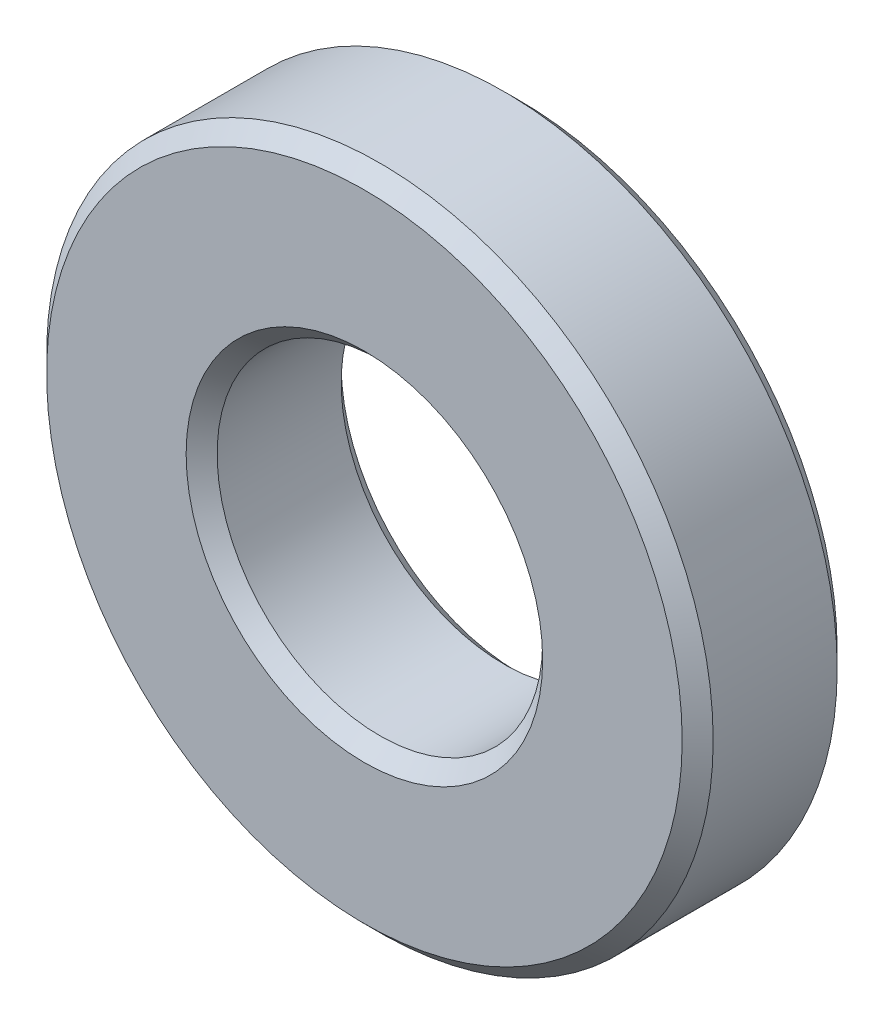
from build123d import *

# Parameters (mm, degrees)
SKETCH1_R           = 10.75
SKETCH1_R_2         = 5.25
BOSS_EXTRUDE1_DEPTH = 5
CHAMFER1_SIZE       = 0.5


with BuildPart() as part:
    # Sketch1 → Boss-Extrude1 (new body)
    with BuildSketch(Plane.XY):
        Circle(SKETCH1_R)
        Circle(SKETCH1_R_2, mode=Mode.SUBTRACT)
    extrude(amount=BOSS_EXTRUDE1_DEPTH)

    # Chamfer1
    chamfer1_edges = [part.edges().sort_by_distance(p)[0] for p in [
        (-10.75, 0, 0),
        (-10.75, 0, 5),
        (-5.25, 0, 0),
        (-5.25, 0, 5),
    ]]
    chamfer(chamfer1_edges, length=CHAMFER1_SIZE)


solid = part.part
